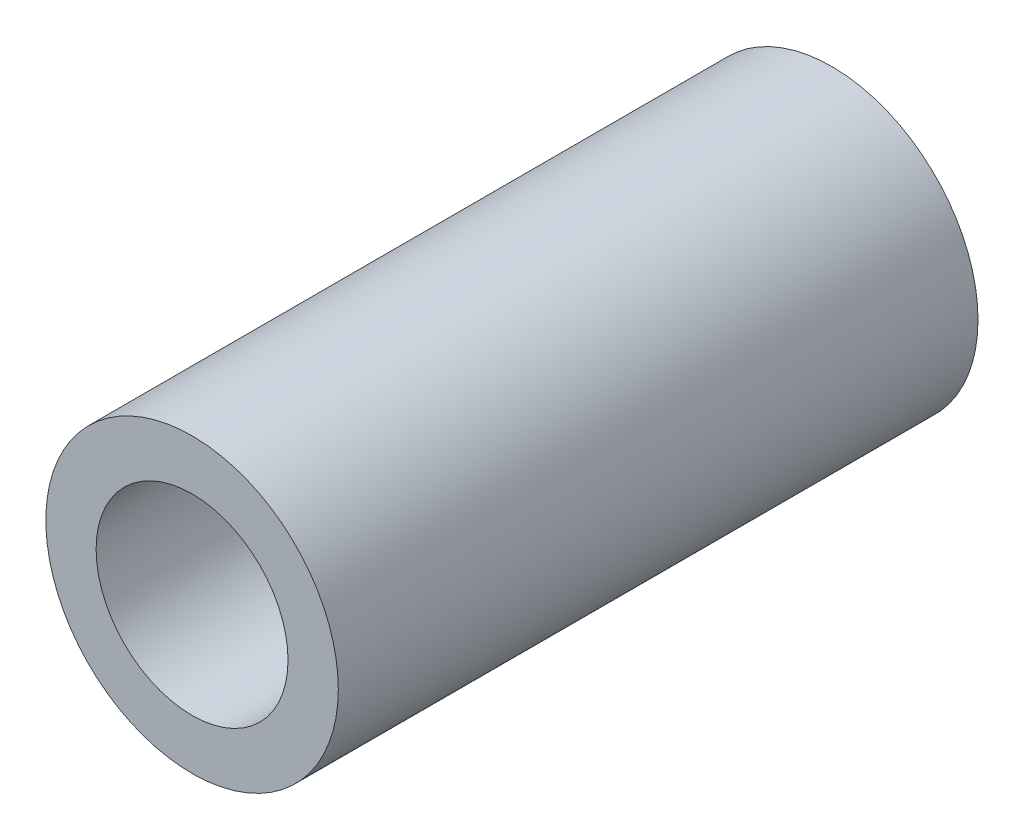
from build123d import *

# Parameters (mm, degrees)
SKETCH1_R                   = 8
BOSS_EXTRUDE1_DEPTH         = 35
M12X1_25_TAPPED_HOLE1_D     = 10.5
M12X1_25_TAPPED_HOLE1_DEPTH = 35
M12X1_25_TAPPED_HOLE1_TIP   = 3.15451825


with BuildPart() as part:
    # Sketch1 → Boss-Extrude1 (new body)
    with BuildSketch(Plane.XY):
        Circle(SKETCH1_R)
    extrude(amount=BOSS_EXTRUDE1_DEPTH)

    # M12x1.25 Tapped Hole1
    with Locations(Plane.XY.offset(35)):
        with Locations((0, 0)):
            Hole(M12X1_25_TAPPED_HOLE1_D / 2, depth=M12X1_25_TAPPED_HOLE1_DEPTH)
            with Locations((0, 0, -(M12X1_25_TAPPED_HOLE1_DEPTH + M12X1_25_TAPPED_HOLE1_TIP / 2))):  # 118° drill point
                Cone(0, M12X1_25_TAPPED_HOLE1_D / 2, M12X1_25_TAPPED_HOLE1_TIP, mode=Mode.SUBTRACT)


solid = part.part
